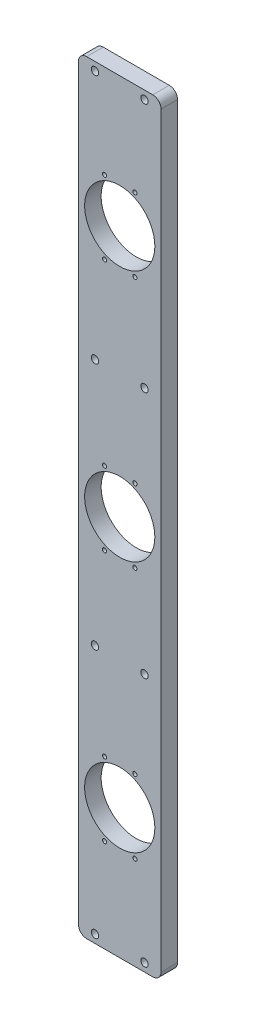
SolidWorks part; units mm, degrees
ref_plane "前视基准面" through (0, 0, 0) normal (0, 0, 1) x (1, 0, 0)
ref_plane "上视基准面" through (0, 0, 0) normal (0, 1, 0) x (1, 0, 0)
ref_plane "右视基准面" through (0, 0, 0) normal (1, 0, 0) x (0, 0, -1)
sketch "草图1" plane through (0, 0, 0) normal (0, 0, 1) x (1, 0, 0)
  line L1 (-50, 462.5) -> (50, 462.5)
  line L2 (-50, 462.5) -> (-50, -462.5)
  line L3 (-50, -462.5) -> (50, -462.5)
  line L4 (50, 462.5) -> (50, -462.5)
  line L5 (-50, 462.5) -> (50, -462.5) construction
  line L6 (-50, -462.5) -> (50, 462.5) construction
  point P0 (0, 0)
  dimension "D1" = 100
  dimension "D2" = 925
extrude "凸台-拉伸1" add sketch "草图1" along normal blind 20
hole_wizard "M6 螺纹孔2" positions "草图10" profile "草图9" tap size "M6" standard "ISO" end condition through all
sketch "草图10" plane through (0, 0, 20) normal (0, 0, 1) x (1, 0, 0)
  line L0 (0, -231.4234) -> (0, -378.7848) construction
  line L1 (0, -305) -> (-18.3688, -260.6538) construction
  line L3 (0, -305) -> (18.3688, -260.6538) construction
  line L4 (63.4467, -305) -> (-56.4425, -305) construction
  line L5 (80.2959, 0) -> (-155.3633, 0) construction
  circle A0 centre (0, -305) radius 48 construction
  point P14 (-18.3688, -260.6538)
  point P17 (18.3688, -260.6538)
  point P21 (18.3688, -349.3462)
  point P22 (-18.3688, -349.3462)
  point P43 (18.3688, 349.3462)
  point P44 (-18.3688, 349.3462)
  point P45 (18.3688, 260.6538)
  point P46 (-18.3688, 260.6538)
  dimension "D2" = 96
  dimension "D1" = 305
  dimension "D3" = 45
sketch "草图9" plane through (-18.3688, -260.6538, 20) normal (1, 0, 0) x (0, -1, 0)
  line L0 (0, 0) -> (0, 20)
  line L1 (0, 20) -> (2.5, 20)
  line L2 (2.5, 20) -> (2.5, 0)
  line L5 (2.5, 0) -> (0, 0)
  line L11 (0, -6.35) -> (0, 107.95) construction
  dimension "通孔螺纹孔钻头直径" = 5
  dimension "通孔螺纹孔钻头深度" = 20
cosmetic thread "孔螺蚊线5" parameters "D2"=6
cosmetic thread "孔螺蚊线6" parameters "D2"=6
cosmetic thread "孔螺蚊线7" parameters "D2"=6
cosmetic thread "孔螺蚊线8" parameters "D2"=6
cosmetic thread "孔螺蚊线9" parameters "D2"=6
cosmetic thread "孔螺蚊线10" parameters "D2"=6
cosmetic thread "孔螺蚊线11" parameters "D2"=6
cosmetic thread "孔螺蚊线12" parameters "D2"=6
sketch "草图11" plane through (0, 0, 20) normal (0, 0, 1) x (1, 0, 0)
  circle A0 centre (0, -305) radius 42.5
  dimension "D1" = 85
  dimension "D2" = 305
extrude "切除-拉伸1" cut sketch "草图11" against normal through all
hole_wizard "M8 六角凹头螺钉的柱形沉头孔2" positions "草图13" profile "草图12" counterbore size "M8" standard "ISO" end condition through all
sketch "草图13" plane through (0, 0, 0) normal (0, 0, -1) x (-1, 0, 0)
  line L1 (-50, -462.5) -> (-50, 462.5) construction
  line L2 (85.785, 0) -> (-83.3714, 0) construction
  point P0 (-30, -452.5)
  point P2 (30, -452.5)
  point P34 (-30, -150)
  point P35 (30, -150)
  point P36 (30, 150)
  point P37 (-30, 150)
  point P38 (30, 452.5)
  point P39 (-30, 452.5)
  dimension "D1" = 60
  dimension "D2" = 905
  dimension "D3" = 20
  dimension "D4" = 2
  dimension "D5" = 300
sketch "草图12" plane through (30, -452.5, 0) normal (1, 0, 0) x (0, 1, 0)
  line L0 (0, 0) -> (0, 20)
  line L1 (0, 20) -> (4.5, 20)
  line L3 (4.5, 20) -> (4.5, 8.6)
  line L4 (4.5, 8.6) -> (7.5, 8.6)
  line L5 (7.5, 8.6) -> (7.5, 0)
  line L7 (7.5, 0) -> (0, 0)
  line L11 (0, -6.35) -> (0, 107.95) construction
  dimension "通孔孔直径" = 9
  dimension "通孔孔深度" = 20
  dimension "柱形沉头孔直径" = 15
  dimension "柱形沉头孔深度" = 8.6
mirror "镜向10" about plane through (0, 0, 0) normal (0, 1, 0) of "切除-拉伸1"
fillet "圆角2" radius 10 4 edges at (-50, 462.5, 10) (50, 462.5, 10) (50, -462.5, 10) (-50, -462.5, 10)
sketch "草图14" plane through (0, 0, 20) normal (0, 0, 1) x (1, 0, 0)
  circle A0 centre (0, 0) radius 42.5
  dimension "D1" = 85
extrude "切除-拉伸2" cut sketch "草图14" against normal through all
hole_wizard "M6 螺纹孔3" positions "草图16" profile "草图15" tap size "M6" standard "ISO" end condition through all
sketch "草图16" plane through (0, 0, 20) normal (0, 0, 1) x (1, 0, 0)
  point P0 (-18.3688, 44.3462)
  point P3 (18.3688, 44.3462)
  point P6 (18.3688, -44.3462)
  point P9 (-18.3688, -44.3462)
sketch "草图15" plane through (-18.3688, 44.3462, 20) normal (1, 0, 0) x (0, -1, 0)
  line L0 (0, 0) -> (0, 20)
  line L1 (0, 20) -> (2.5, 20)
  line L2 (2.5, 20) -> (2.5, 0)
  line L5 (2.5, 0) -> (0, 0)
  line L11 (0, -6.35) -> (0, 107.95) construction
  dimension "通孔螺纹孔钻头直径" = 5
  dimension "通孔螺纹孔钻头深度" = 20
cosmetic thread "孔螺蚊线13" parameters "D2"=6
cosmetic thread "孔螺蚊线14" parameters "D2"=6
cosmetic thread "孔螺蚊线15" parameters "D2"=6
cosmetic thread "孔螺蚊线16" parameters "D2"=6
